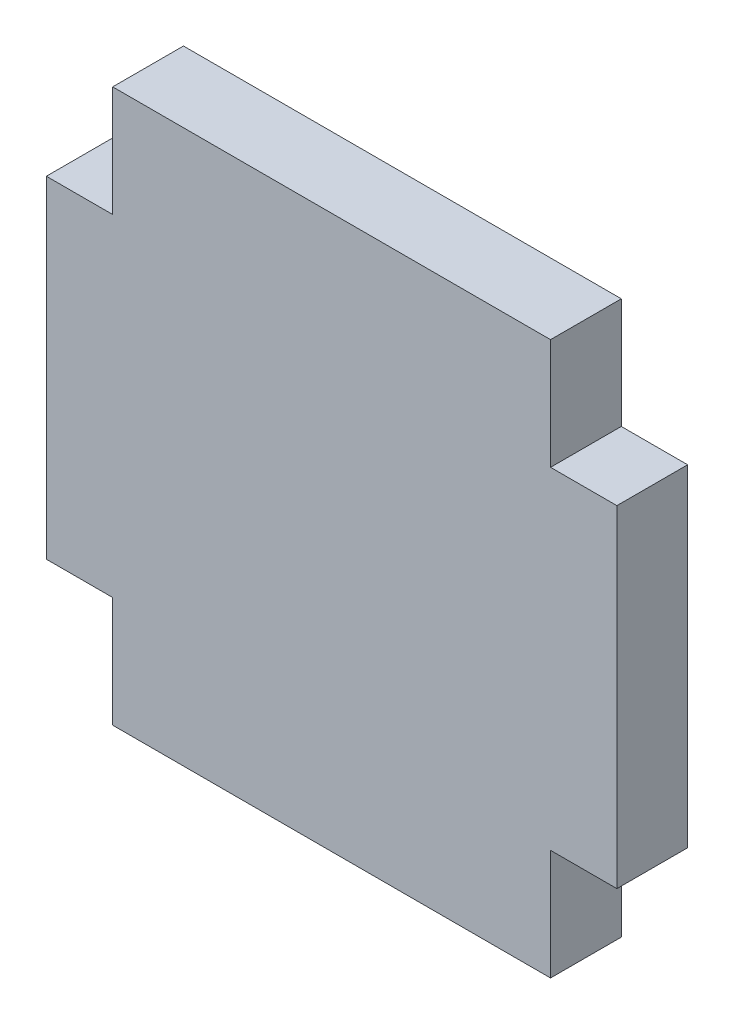
SolidWorks part; units mm, degrees
material "SPHC"
ref_plane "Front Plane" through (0, 0, 0) normal (0, 0, 1) x (1, 0, 0)
ref_plane "Top Plane" through (0, 0, 0) normal (0, 1, 0) x (1, 0, 0)
ref_plane "Right Plane" through (0, 0, 0) normal (1, 0, 0) x (0, 0, -1)
sketch "Sketch1" plane through (0, 0, 0) normal (0, 0, 1) x (1, 0, 0)
  line L0 (30.5, 25) -> (50.3, 25)
  line L2 (50.3, 72.5) -> (50.3, -82.5) construction
  line L3 (50.3, 25) -> (50.3, 30)
  line L4 (50.3, 50) -> (30.5, 50)
  line L5 (30.5, 50) -> (30.5, 45)
  line L6 (30.5, 30) -> (27.5, 30)
  line L7 (27.5, 30) -> (27.5, 45)
  line L8 (27.5, 45) -> (30.5, 45)
  line L9 (30.5, 30) -> (30.5, 25)
  line L10 (50.3, 30) -> (53.3, 30)
  line L11 (53.3, 30) -> (53.3, 45)
  line L12 (53.3, 45) -> (50.3, 45)
  line L13 (50.3, 45) -> (50.3, 50)
  dimension "D1" = 25
  dimension "D2" = 15
  dimension "D3" = 5
  dimension "D4" = 3
  dimension "D5" = 15
  dimension "D6" = 3
extrude "Boss-Extrude1" add sketch "Sketch1" along normal mid plane 3.2
